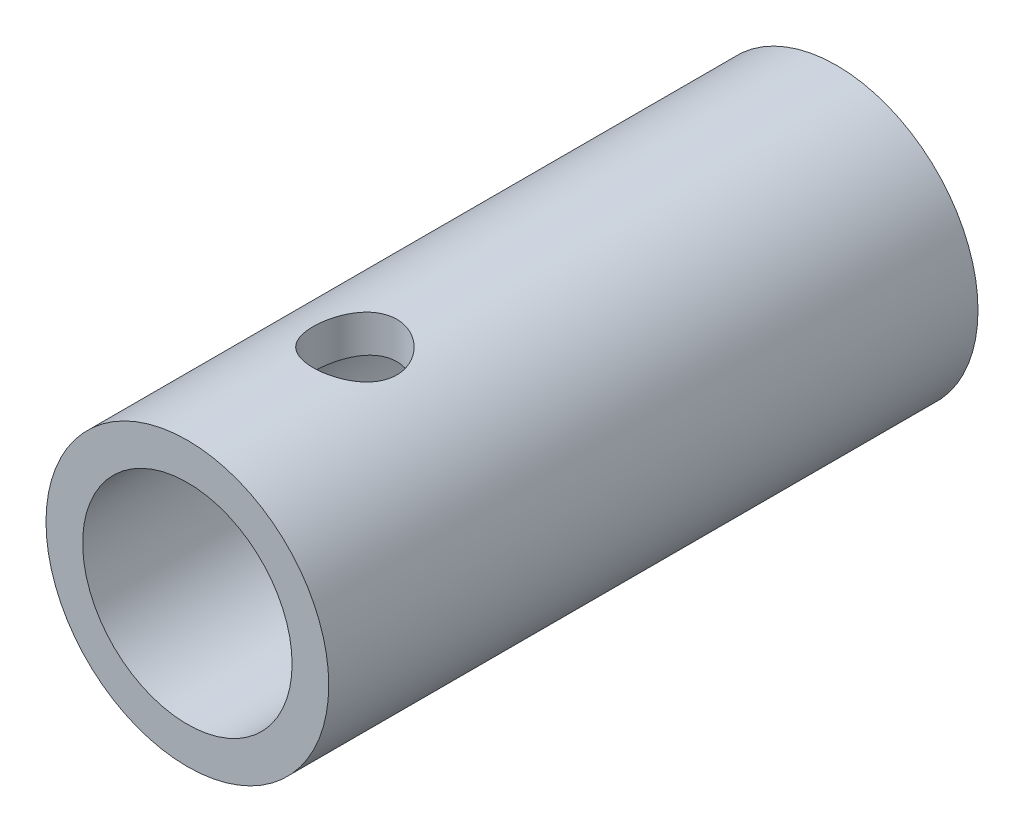
SolidWorks part; units mm, degrees
ref_plane "Front Plane" through (0, 0, 0) normal (0, 0, 1) x (1, 0, 0)
ref_plane "Top Plane" through (0, 0, 0) normal (0, 1, 0) x (1, 0, 0)
ref_plane "Right Plane" through (0, 0, 0) normal (1, 0, 0) x (0, 0, -1)
sketch "Sketch1" plane through (0, 0, 0) normal (0, 0, 1) x (1, 0, 0)
  circle A0 centre (0, 0) radius 13.5
  circle A1 centre (0, 0) radius 10
  dimension "D1" = 27
  dimension "D2" = 20
extrude "Boss-Extrude1" add sketch "Sketch1" against normal blind 62
sketch "Sketch2" plane through (0, 0, 0) normal (0, 1, 0) x (1, 0, 0)
  circle A0 centre (0, 16) radius 4
  dimension "D1" = 8
  dimension "D2" = 16
extrude "Cut-Extrude1" cut sketch "Sketch2" along normal blind 62
